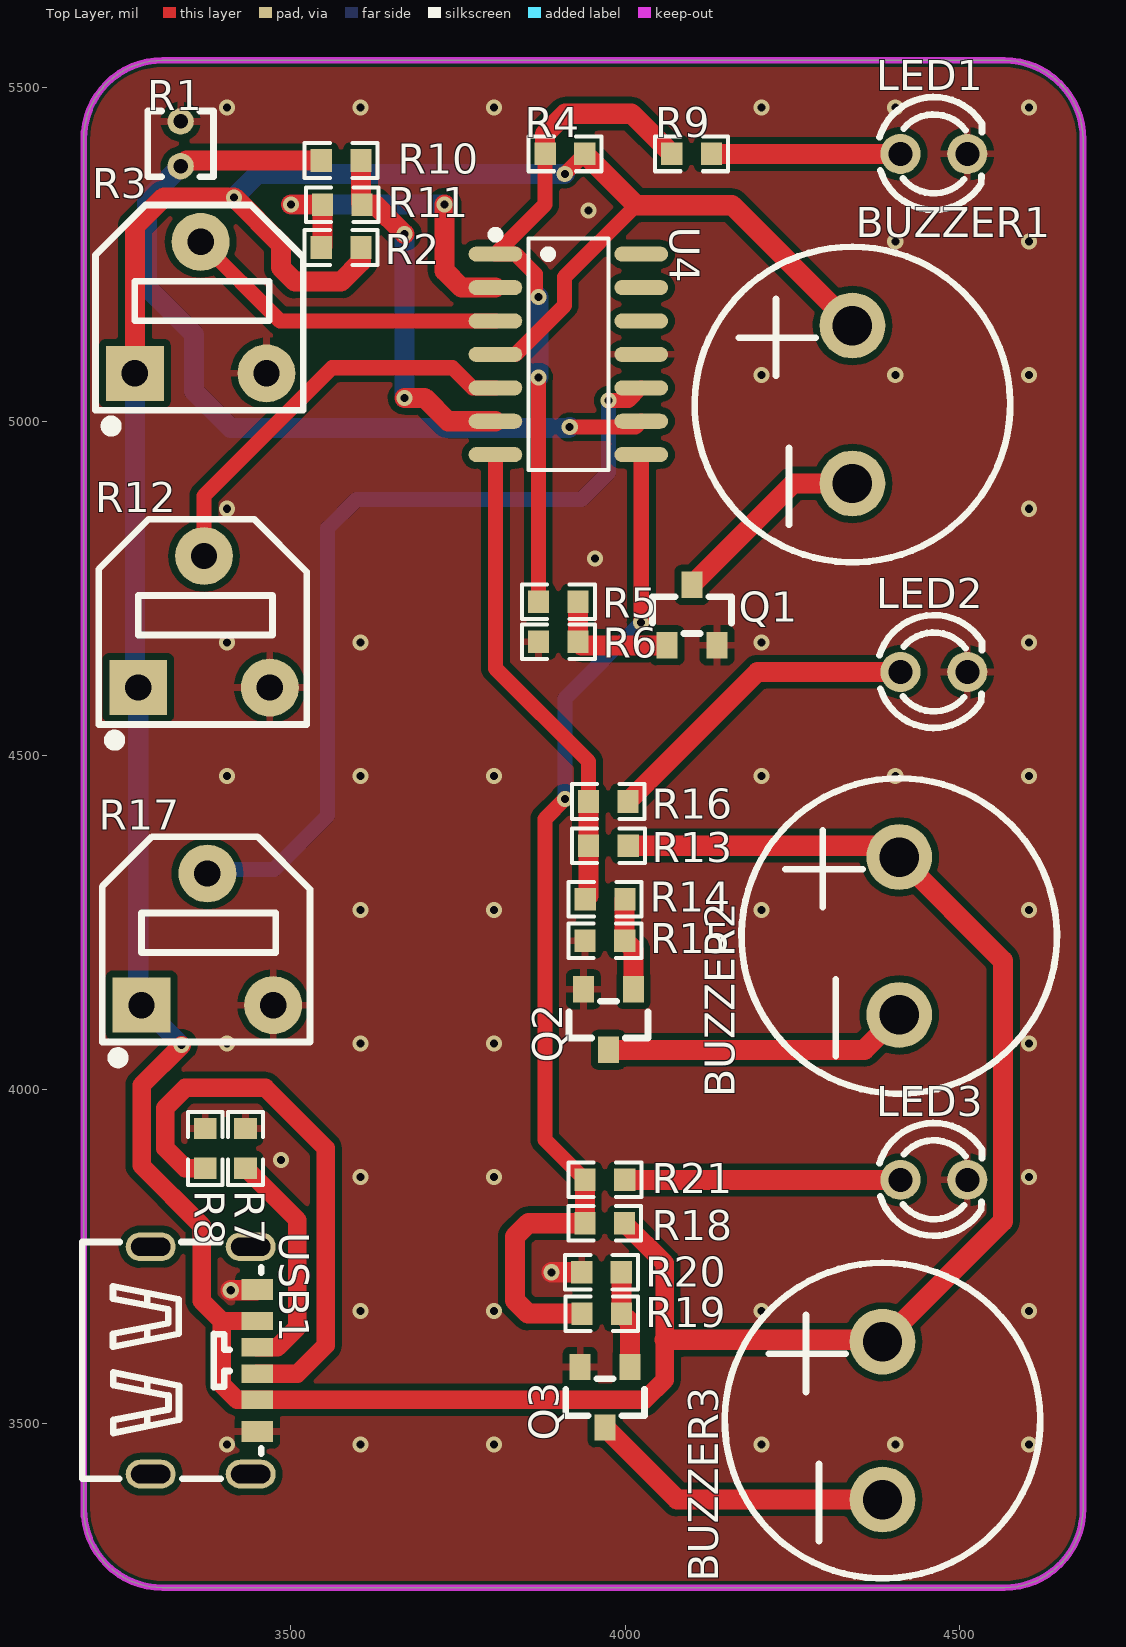
[diagram p0: Top Layer view]
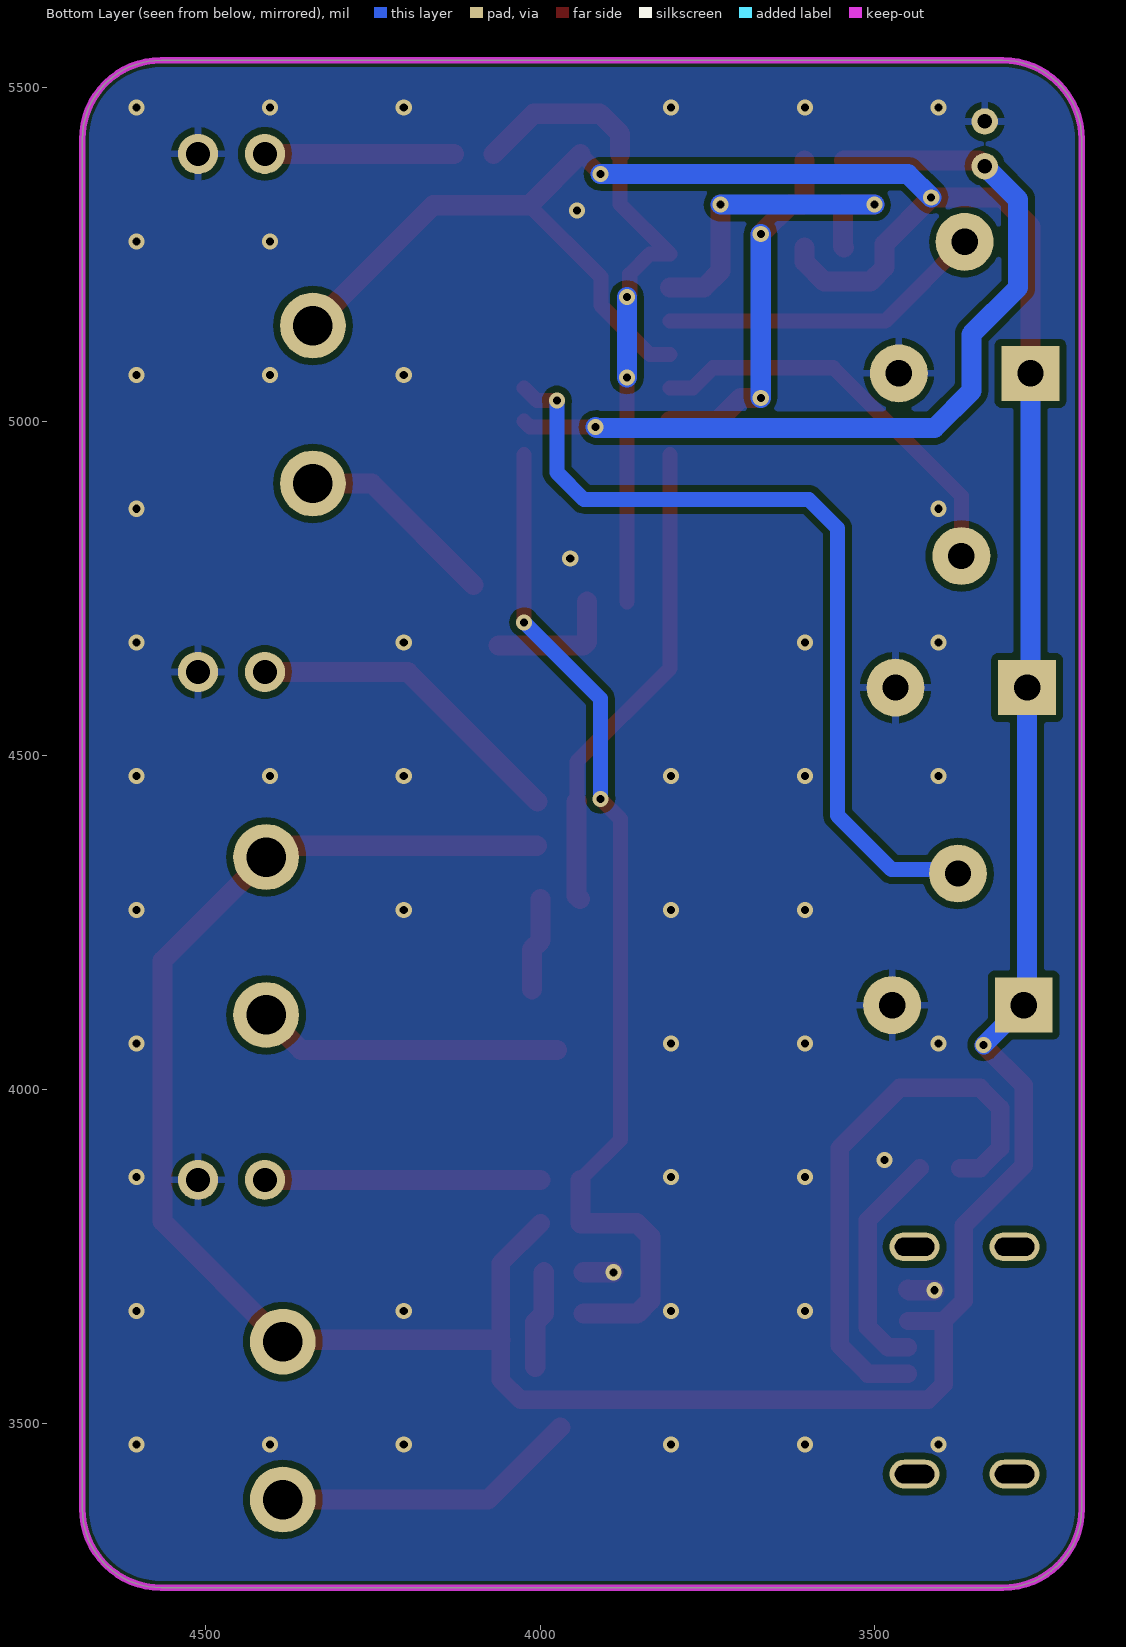
[diagram p1: Bottom Layer view, seen from below]
# Altium PCB MISC51921.pcbdoc
Units mil, origin at the board's own origin, x right, y up, seen from the top; angles counter-clockwise.
Board outline 1495 x 2285 mil, 2 copper layers (Top Layer, Bottom Layer), stack 62.206 mil thick; 32 components, 22 nets, 90 pads, 62 vias.

## Layer stack, top to bottom
Top Solder Mask Layer: solder mask 0.394, Dk 3.3
Top Layer: signal copper 1.379
Dielectric1: surface 59.449, FR4, Dk 4.5
Bottom Layer: signal copper 1.378
Bottom Solder Mask Layer: solder mask 0.394, Dk 3.3

## Board outline
3308.11,5540 ccw(c3308.11,5421.89) 3190,5421.89 3190,3373.11 ccw(c3308.11,3373.11) 3308.11,3255 4566.89,3255 ccw(c4566.89,3373.11) 4685,3373.11 4685,5421.89 ccw(c4566.89,5421.89) 4566.89,5540

## Design rules (kind name [scope] priority, off if disabled: settings)
BoardOutlineClearance copperThickness2oz_1 [All] p2 off: genericclearance=7.99 ignorepadtopadclearanceinfootprint=FALSE except(0: Arc-SplitContinuation Track-SplitContinuation SMDPad-SplitContinuation THPad-SplitContinuation Via-SplitContinuation Fill-SplitContinuation Region-SplitContinuation Poly-SplitContinuation Text-SplitContinuation Hole-SplitContinuation; 5.98: Arc-CutoutEdge Track-CutoutEdge SMDPad-CutoutEdge THPad-CutoutEdge Via-CutoutEdge Text-CutoutEdge; 6.89: Hole-OutlineEdge Hole-CutoutEdge; 10: Poly-OutlineEdge Poly-CutoutEdge; 11.81: Arc-OutlineEdge Track-OutlineEdge SMDPad-OutlineEdge THPad-OutlineEdge Via-OutlineEdge Fill-OutlineEdge Region-OutlineEdge Text-OutlineEdge Fill-CutoutEdge Region-CutoutEdge)
BoardOutlineClearance Plane_innerPlane_1 [All] p4 off: genericclearance=4.02 ignorepadtopadclearanceinfootprint=FALSE except(0: Arc-SplitContinuation Track-SplitContinuation SMDPad-SplitContinuation THPad-SplitContinuation Via-SplitContinuation Fill-SplitContinuation Region-SplitContinuation Poly-SplitContinuation Text-SplitContinuation Hole-SplitContinuation; 5.98: Arc-CutoutEdge Track-CutoutEdge SMDPad-CutoutEdge THPad-CutoutEdge Via-CutoutEdge Text-CutoutEdge; 6.89: Hole-OutlineEdge Hole-CutoutEdge; 10: Poly-OutlineEdge Poly-CutoutEdge; 11.81: Arc-OutlineEdge Track-OutlineEdge SMDPad-OutlineEdge THPad-OutlineEdge Via-OutlineEdge Fill-OutlineEdge Region-OutlineEdge Text-OutlineEdge Fill-CutoutEdge Region-CutoutEdge)
BoardOutlineClearance Copper_copperRegion_1 [All] p6 off: genericclearance=4.02 ignorepadtopadclearanceinfootprint=FALSE except(0: Arc-SplitContinuation Track-SplitContinuation SMDPad-SplitContinuation THPad-SplitContinuation Via-SplitContinuation Fill-SplitContinuation Region-SplitContinuation Poly-SplitContinuation Text-SplitContinuation Hole-SplitContinuation; 5.98: Arc-CutoutEdge Track-CutoutEdge SMDPad-CutoutEdge THPad-CutoutEdge Via-CutoutEdge Text-CutoutEdge; 6.89: Hole-OutlineEdge Hole-CutoutEdge; 10: Poly-OutlineEdge Poly-CutoutEdge; 11.81: Arc-OutlineEdge Track-OutlineEdge SMDPad-OutlineEdge THPad-OutlineEdge Via-OutlineEdge Fill-OutlineEdge Region-OutlineEdge Text-OutlineEdge Fill-CutoutEdge Region-CutoutEdge)
BoardOutlineClearance copperThickness1oz_1 [All] p8: genericclearance=4.02 ignorepadtopadclearanceinfootprint=FALSE except(0: Arc-SplitContinuation Track-SplitContinuation SMDPad-SplitContinuation THPad-SplitContinuation Via-SplitContinuation Fill-SplitContinuation Region-SplitContinuation Poly-SplitContinuation Text-SplitContinuation Hole-SplitContinuation; 5.98: Arc-CutoutEdge Track-CutoutEdge SMDPad-CutoutEdge THPad-CutoutEdge Via-CutoutEdge Text-CutoutEdge; 6.89: Hole-OutlineEdge Hole-CutoutEdge; 10: Poly-OutlineEdge Poly-CutoutEdge; 11.81: Arc-OutlineEdge Track-OutlineEdge SMDPad-OutlineEdge THPad-OutlineEdge Via-OutlineEdge Fill-OutlineEdge Region-OutlineEdge Text-OutlineEdge Fill-CutoutEdge Region-CutoutEdge)
Clearance copperThickness2oz [All] p1 off: gap=7.99 ignorepadtopadclearanceinfootprint=FALSE except(5.98: SMDPad-Track SMDPad-SMDPad THPad-Track SMDPad-THPad THPad-THPad Track-Via SMDPad-Via THPad-Via Via-Via Fill-SMDPad Region-SMDPad Fill-THPad Region-THPad Fill-Via Region-Via Fill-Fill Fill-Region Region-Region Arc-Track Arc-SMDPad Arc-THPad Arc-Via Fill-Arc Region-Arc Arc-Arc Text-Track SMDPad-Text Text-THPad Text-Via Fill-Text Region-Text Arc-Text Text-Text; 6.89: Hole-Track Hole-SMDPad Hole-THPad Hole-Via Fill-Hole Region-Hole Hole-Arc Hole-Text; 10: Poly-Track Poly-SMDPad Poly-THPad Poly-Via Poly-Fill Poly-Region Poly-Poly Poly-Arc Poly-Text Poly-Hole; 11.81: Fill-Track Region-Track)
Clearance Plane_innerPlane [All] p3 off: gap=4.02 ignorepadtopadclearanceinfootprint=FALSE except(5.98: SMDPad-Track SMDPad-SMDPad THPad-Track SMDPad-THPad THPad-THPad Track-Via SMDPad-Via THPad-Via Via-Via Fill-SMDPad Region-SMDPad Fill-THPad Region-THPad Fill-Via Region-Via Fill-Fill Fill-Region Region-Region Arc-Track Arc-SMDPad Arc-THPad Arc-Via Fill-Arc Region-Arc Arc-Arc Text-Track SMDPad-Text Text-THPad Text-Via Fill-Text Region-Text Arc-Text Text-Text; 6.89: Hole-Track Hole-SMDPad Hole-THPad Hole-Via Fill-Hole Region-Hole Hole-Arc Hole-Text; 10: Poly-Track Poly-SMDPad Poly-THPad Poly-Via Poly-Fill Poly-Region Poly-Poly Poly-Arc Poly-Text Poly-Hole; 11.81: Fill-Track Region-Track)
Clearance Copper_copperRegion [All] p5 off: gap=4.02 ignorepadtopadclearanceinfootprint=FALSE except(5.98: SMDPad-Track SMDPad-SMDPad THPad-Track SMDPad-THPad THPad-THPad Track-Via SMDPad-Via THPad-Via Via-Via Fill-SMDPad Region-SMDPad Fill-THPad Region-THPad Fill-Via Region-Via Fill-Fill Fill-Region Region-Region Arc-Track Arc-SMDPad Arc-THPad Arc-Via Fill-Arc Region-Arc Arc-Arc Text-Track SMDPad-Text Text-THPad Text-Via Fill-Text Region-Text Arc-Text Text-Text; 6.89: Hole-Track Hole-SMDPad Hole-THPad Hole-Via Fill-Hole Region-Hole Hole-Arc Hole-Text; 10: Poly-Track Poly-SMDPad Poly-THPad Poly-Via Poly-Fill Poly-Region Poly-Poly Poly-Arc Poly-Text Poly-Hole; 11.81: Fill-Track Region-Track)
Clearance copperThickness1oz [All] p7: gap=4.02 ignorepadtopadclearanceinfootprint=FALSE except(5.98: SMDPad-Track SMDPad-SMDPad THPad-Track SMDPad-THPad THPad-THPad Track-Via SMDPad-Via THPad-Via Via-Via Fill-SMDPad Region-SMDPad Fill-THPad Region-THPad Fill-Via Region-Via Fill-Fill Fill-Region Region-Region Arc-Track Arc-SMDPad Arc-THPad Arc-Via Fill-Arc Region-Arc Arc-Arc Text-Track SMDPad-Text Text-THPad Text-Via Fill-Text Region-Text Arc-Text Text-Text; 6.89: Hole-Track Hole-SMDPad Hole-THPad Hole-Via Fill-Hole Region-Hole Hole-Arc Hole-Text; 10: Poly-Track Poly-SMDPad Poly-THPad Poly-Via Poly-Fill Poly-Region Poly-Poly Poly-Arc Poly-Text Poly-Hole; 11.81: Fill-Track Region-Track)
DiffPairsRouting differentialPair [All] p1: maxlimit=6 minlimit=6 mostfreqgap=6 toplayer_minwidth=5 toplayer_prefwidth=10 toplayer_maxwidth=100 toplayer_mingap=6 toplayer_prefgap=6 toplayer_maxgap=6 bottomlayer_minwidth=5 bottomlayer_prefwidth=10 bottomlayer_maxwidth=100 bottomlayer_mingap=6 bottomlayer_prefgap=6 bottomlayer_maxgap=6 maxuncoupledlength=10
HoleToHoleClearance otherClearance [All] p1: gap=11.81 allowstackedmicrovias=TRUE
Length netLength [All] p1: minlimit=0 maxlimit=0
PasteMaskExpansion pasteMaskExpansion [All] p1: expansion=0
PlaneConnect innerPlane [All] p1: planeconnectstyle=Relief reliefexpansion=20 reliefentries=4 reliefconductorwidth=10 reliefairgap=10
PolygonConnect copperRegion [All] p1: connectstyle=Relief reliefconductorwidth=10 reliefentries=4 polygonreliefangle="90 Angle" airgapwidth=10 via.connectstyle=Relief via.reliefconductorwidth=10 via.reliefentries=4 via.polygonreliefangle="90 Angle" via.airgapwidth=10
RoutingVias viaSize [All] p1: holewidth=12.01 width=24.02 viastyle="Through Hole" minholewidth=11.81 minwidth=19.68 maxholewidth=248.03 maxwidth=393.7
SolderMaskExpansion solderMaskExpansion [IsVia] p1: expansion=-1000 istentingtop=TRUE
SolderMaskExpansion solderMaskExpansion [All] p2: expansion=2.01 istentingtop=FALSE
Width copperThickness2oz_2 [All] p1 off: maxlimit=100 minlimit=8 preferedwidth=10
Width copperThickness1oz_2 [All] p2: maxlimit=100 minlimit=5 preferedwidth=30

## Components (designator, comment, footprint, x,y, rotation, side; value= is the part's Value field where it differs from the comment)
BUZZER1 "buzzer" BUZ-TH_BD12.0-P6.00-D0.9-RD 4340,5025 r90 top
BUZZER2 "buzzer" BUZ-TH_BD12.0-P6.00-D0.9-RD 4410,4230 r90 top
BUZZER3 "buzzer" BUZ-TH_BD12.0-P6.00-D0.9-RD 4385,3505 r90 top
LED1 "" LED_TH-3mm 4461.85,5400 r0 top
LED2 "" LED_TH-3mm 4461.85,4625 r0 top
LED3 "" LED_TH-3mm 4461.85,3865.22 r0 top
Q1 "" S8050_SOT-23 4095,4710 r270 top
Q2 "" S8050_SOT-23 3980,4105 r90 top
Q3 "" S8050_SOT-23 3975,3540 r90 top
R1 "MF52A503F3950 (A1)" RES-TH_L2.5-W2.5-P1.70-D0.3 3335,5415 r270 top
R2 "1K" R0603 3575,5260 r0 top
R3 "10kΩ" RES-ADJ-SMD_RM065-V1 3365,5170 r0 top
R4 "10K" R0603 3910,5400 r0 top
R5 "1K" R0603 3900,4730 r180 top
R6 "10K" R0603 3900,4670 r180 top
R7 "5.1K" R0603 3431.98,3912.32 r270 top
R8 "5.1K" R0603 3371.98,3912.32 r270 top
R9 "100" R0603 4099.32,5400 r180 top
R10 "1K" R0603 3575,5390 r0 top
R11 "1K" R0603 3576.75,5324.04 r180 top
R12 "10kΩ" RES-ADJ-SMD_RM065-V1 3370,4700 r0 top
R13 "10K" R0603 3975,4365 r0 top
R14 "1K" R0603 3970,4285 r180 top
R15 "10K" R0603 3969.67,4222.97 r180 top
R16 "100" R0603 3974.67,4431.29 r180 top
R17 "10kΩ" RES-ADJ-SMD_RM065-V1 3375,4225 r0 top
R18 "10K" R0603 3969.5,3800.27 r0 top
R19 "1K" R0603 3965,3665 r180 top
R20 "10K" R0603 3964.67,3726.91 r180 top
R21 "100" R0603 3969.67,3865.22 r180 top
U4 "LM324DT" SOIC-14_L8.7-W3.9-P1.27-LS6.0-BL 3915,5100 r270 top
USB1 "TYPE-C-6P-DIP2X2" TYPE-C-SMD_TYPE-C-6P 3370,3595 r270 top

## Footprints (in the part's own frame and the unit in brackets; to place one, negate y for a bottom-side part, rotate by r counter-clockwise, add the part's x,y. Pads: shape width x height; smd on the part's side, far side on the other; paste and mask are expansions set on the pad)
BUZ-TH_BD12.0-P6.00-D0.9-RD [mm]
  round 2.5 hole 1.5 paste+0 mask+0.05: 1(-3,0) 2(3,0)
  silkscreen extent -5.99,-5.99 5.99,5.99
LED_TH-3mm [mil]
  round 60 hole 36 paste+0 mask+2: 1(-50,0) 2(50,0)
  silkscreen extent -81,-84 72,85
R0603 [mil]
  rect 31.75x34.02 smd paste-3937.01 mask+2: 1(-29.66,0) 2(29.66,0)
  silkscreen extent -55,-26 55,26
RES-ADJ-SMD_RM065-V1 [mm]
  rect 2.2x2.1 hole 1 paste+0 mask+0.05: 1(-2.5,-2.5)
  round 2.2 hole 1 paste+0 mask+0.05: 2(0,2.5) 3(2.5,-2.5)
  silkscreen extent -4,-4.7 3.9,3.9
RES-TH_L2.5-W2.5-P1.70-D0.3 [mm]
  round 1 hole 0.55: 1(-0.85,0) 2(0.85,0)
  silkscreen extent -1.25,-1.25 1.25,1.25
S8050_SOT-23 [mm]
  rect 1x0.8 smd paste+0 mask+0.051: 1(1.15,-0.823) 2(1.15,1.077) 3(-1.15,0.127)
  silkscreen extent -0.7,-1.37 0.7,1.63
SOIC-14_L8.7-W3.9-P1.27-LS6.0-BL [mil]
  oval 22.6x80.24 smd: 1(-150,-109.02) 2(-100,-109.02) 3(-50,-109.02) 4(0,-109.02) 5(50,-109.02) 6(100,-109.02) 7(150,-109.02) 8(150,109.02) 9(100,109.02) 10(50,109.02) 11(0,109.02) 12(-50,109.02) 13(-100,109.02) 14(-150,109.02)
  silkscreen extent -185,-115 173,60
TYPE-C-SMD_TYPE-C-6P [mm]
  oval 1.1x1.9 hole 0.7 slot 1.5 at 90 deg: 7(-4.32,1.775) 7(-4.32,-2.025) 7(4.32,1.775) 7(4.32,-2.025)
  rect 0.7x1.2 smd paste-100 mask+0.051: A5(-0.5,2.025) A9(1.5,2.025) B5(0.5,2.025) B9(-1.5,2.025)
  rect 0.8x1.2 smd paste-100 mask+0.051: A12(2.7,2.025) B12(-2.7,2.025)
  silkscreen extent -4.5,-4.63 4.5,2.18

## Via types
v1: diameter 24.02, hole 12, Top Layer to Bottom Layer, 60 vias
v2: diameter 24, hole 12, Top Layer to Bottom Layer, 2 vias

## Nets (pads, with @x,y where several pads share a name; then routed paths per layer and width w, separated by ;. In a path a pad name is that pad's centre, name@x,y a point inside that pad or via, vN(x,y) a via of type N, cw(c..) or ccw(c..) an arc to the next point about the centre after c; other vN are vias at no path point)
$1N355: R3.2 U4.3 | length 490
  Top Layer w22.6: R3.2 3483.43,5150 U4.3
$1N794: Q1.1 R5.1 R6.1 | length 195.1
  Top Layer w30: R5.1 R6.1 3934.94,4664.72 Q1.1
$1N950: BUZZER1.1 Q1.3 | length 302.8
  Top Layer w30: Q1.3 4251.62,4906.89 BUZZER1.1
$1N1367: R7.2 USB1.A5 | length 342.6
  Top Layer w27.56: R7.2 3509.72,3804.91 3509.72,3644.68 3479.72,3614.68 USB1.A5
$1N1371: R8.2 USB1.B5 | length 837
  Top Layer w27.56: R8.2 3341.98,3882.66 3311.98,3912.66 3311.98,3972.66 3341.98,4002.66 3461.98,4002.66 3551.98,3912.66 3551.98,3617.57 3509.72,3575.32 USB1.B5
$1N1474: LED1.1 R9.1 | length 282.9
  Top Layer w30: R9.1 LED1.1
$1N1480: R4.1 R5.2 R9.2 U4.1 | length 1001.6
  Top Layer w22.6: R5.2 v1(3870.34,5065.64) ; v1(3870.34,5185.64) 3865.98,5190 3865.98,5220 3835.98,5250 U4.1 3880.34,5324.36 R4.1
  Top Layer w30: R4.1 3880.34,5430 3910.34,5460 4009.66,5460 R9.2
  Bottom Layer w30: v1(3870.34,5065.64) v1(3870.34,5185.64)
$1N1507: R1.2 R10.1 U4.9 | length 1296
  Top Layer w22.6: v1(3917.09,4991.34) 4015.36,4991.34 U4.9
  Top Layer w30: R1.2 3343.47,5390 R10.1
  Bottom Layer w30: R1.2 3285,5331.53 3285,5200 3355,5130 3355,5045 3410,4990 3915.75,4990 v1(3917.09,4991.34)
$1N1538: R10.2 R11.1 U4.6 | length 544
  Top Layer w30: R10.2 3604.66,5325.79 R11.1 3625.96,5324.04 v1(3670,5280) ; v1(3670,5035) 3700,5035 3735,5000 U4.6
  Bottom Layer w30: v1(3670,5035) v1(3670,5280)
$1N1542: R2.1 R11.2 U4.2 | length 527.2
  Top Layer w30: v1(3500,5324.04) R11.2 3547.09,5261.75 R2.1 ; v1(3730,5324.04) 3730,5225 3755,5200 U4.2
  Bottom Layer w30: v1(3500,5324.04) v1(3730,5324.04)
$1N1906: R12.2 U4.5 | length 617.8
  Top Layer w22.6: R12.2 3370,4888.43 3561.57,5080 3741.57,5080 3771.57,5050 U4.5
$1N1923: Q2.1 R14.1 R15.1 | length 140.3
  Top Layer w30: R14.1 3999.33,4284.67 R15.1 4012.4,4209.91 Q2.1
$1N1930: BUZZER2.1 Q2.3 | length 456.6
  Top Layer w30: Q2.3 4357.83,4059.72 BUZZER2.1
$1N1934: LED2.1 R16.1 | length 487.8
  Top Layer w30: R16.1 4198.05,4625 LED2.1
$1N1936: R13.1 R14.2 R16.2 U4.7 | length 724.8
  Top Layer w22.6: U4.7 3805.98,4630.32 3945.01,4491.29 R16.2
  Top Layer w30: R14.2 3945.34,4290 R13.1 3945.34,4430.96 R16.2
$1N2311: R17.2 U4.10 | length 1264.9
  Top Layer w22.6: v1(3975,5030.98) 4005,5030.98 U4.10
  Bottom Layer w22.6: R17.2 3381.19,4329.61 3474.61,4329.61 3555,4410 3555,4840 3598.14,4883.14 3934.72,4883.14 3975,4923.43 v1(3975,5030.98)
$1N2328: Q3.1 R19.1 R20.1 | length 147
  Top Layer w30: R20.1 3994.66,3726.58 R19.1 4007.4,3652.26 Q3.1
$1N2335: BUZZER3.1 Q3.3 | length 459.7
  Top Layer w30: Q3.3 4077.83,3386.89 BUZZER3.1
$1N2339: LED3.1 R21.1 | length 412.5
  Top Layer w30: R21.1 LED3.1
$1N2341: R18.1 R19.2 R21.2 U4.8 | length 1551
  Top Layer w22.6: v1(3910.01,4435.22) 3880.01,4405.22 3880.01,3925.22 R21.2 ; v1(4024.02,4699.22) U4.8
  Top Layer w30: R19.2 3854.86,3665 3835,3684.86 3835,3780 3855.27,3800.27 R18.1 R21.2@3939.84,3865.05
  Bottom Layer w22.6: v1(3910.01,4435.22) 3910.01,4585.22 v1(4024.02,4699.22)
GND: LED1.2 LED2.2 LED3.2 Q1.2 Q2.2 Q3.2 R1.1 R3.3 R6.2 R7.1 R8.1 R12.3 R15.2 R17.3 R20.2 U4.11 USB1.A12 USB1.B12 | length 85.3
  Top Layer w30: v2(3410,3700) 3448.43,3700 USB1.B12 ; v2(3890,3726.91) R20.2
  other v1: 3404.1,3469.1 3604.1,3469.1 3804.1,3469.1 4204.1,3469.1 4404.1,3469.1 4604.1,3469.1 3604.1,3669.1 3804.1,3669.1 4204.1,3669.1 4604.1,3669.1 3604.1,3869.1 3804.1,3869.1 4604.1,3869.1 3485,3895 3404.1,4069.1 3604.1,4069.1 3804.1,4069.1 4604.1,4069.1 3604.1,4269.1 3804.1,4269.1 4204.1,4269.1 4604.1,4269.1 3404.1,4469.1 3604.1,4469.1 3804.1,4469.1 4204.1,4469.1 4404.1,4469.1 4604.1,4469.1 3404.1,4669.1 3604.1,4669.1 4204.1,4669.1 4604.1,4669.1 3955,4795 3404.1,4869.1 4604.1,4869.1 4204.1,5069.1 4404.1,5069.1 4604.1,5069.1 4404.1,5269.1 4604.1,5269.1 3945,5315 3404.1,5469.1 3604.1,5469.1 3804.1,5469.1 4204.1,5469.1 4404.1,5469.1 4604.1,5469.1
VCC: BUZZER1.2 BUZZER2.2 BUZZER3.2 R2.2 R3.1 R4.2 R12.1 R13.2 R17.1 R18.2 U4.4 USB1.A9 USB1.B9 | length 6285
  Top Layer w22.6: U4.4 3835.98,5100 3909.09,5173.11 3909.09,5215.65 4016.55,5323.11 ; v1(3909.66,5370) R4.2
  Top Layer w27.56: v1(3336.57,4066.57) 3276.57,4006.57 3276.57,3886.57 3366.57,3796.57 3366.57,3684.05 3396.57,3654.05 ; USB1.B9 3396.57,3654.05 ; R18.2 4059.16,3740.27 4059.16,3625.95 4059.16,3565.95 4029.16,3535.95 USB1.A9 3419.72,3535.95 3396.57,3559.09 3396.57,3654.05
  Top Layer w30: R3.1 3266.57,5291.57 3310,5335 v1(3415,5335) 3485,5265 3485,5230 3506.21,5208.79 3575,5208.79 3604.66,5238.45 R2.2 ; R4.2 4016.55,5323.11 4160,5323.11 BUZZER1.2 ; R13.2 4393.11,4365 BUZZER2.2 4565,4193.11 4565,3803.11 BUZZER3.2 4382.16,3625.95 4059.16,3625.95
  Bottom Layer w27.56: R17.1 v1(3336.57,4066.57)
  Bottom Layer w30: R3.1 3266.57,4606.57 R12.1 3271.57,4131.57 R17.1 ; v1(3415,5335) 3450,5370 v1(3909.66,5370)
pads on no net: U4.12 U4.13 U4.14 USB1.7

## Polygon pours and split planes (outlines as drawn)
GND on Top Layer (solid, remove dead copper, pour order 0): 3040,5625 3040,3205 4900,3205 4900,5625
GND on Bottom Layer (solid, remove dead copper, pour order 2): 3000,5740 3000,3000 4870,3000 4870,5740

## Keep-outs
Board Outline Layer:
  the board outline again, w10